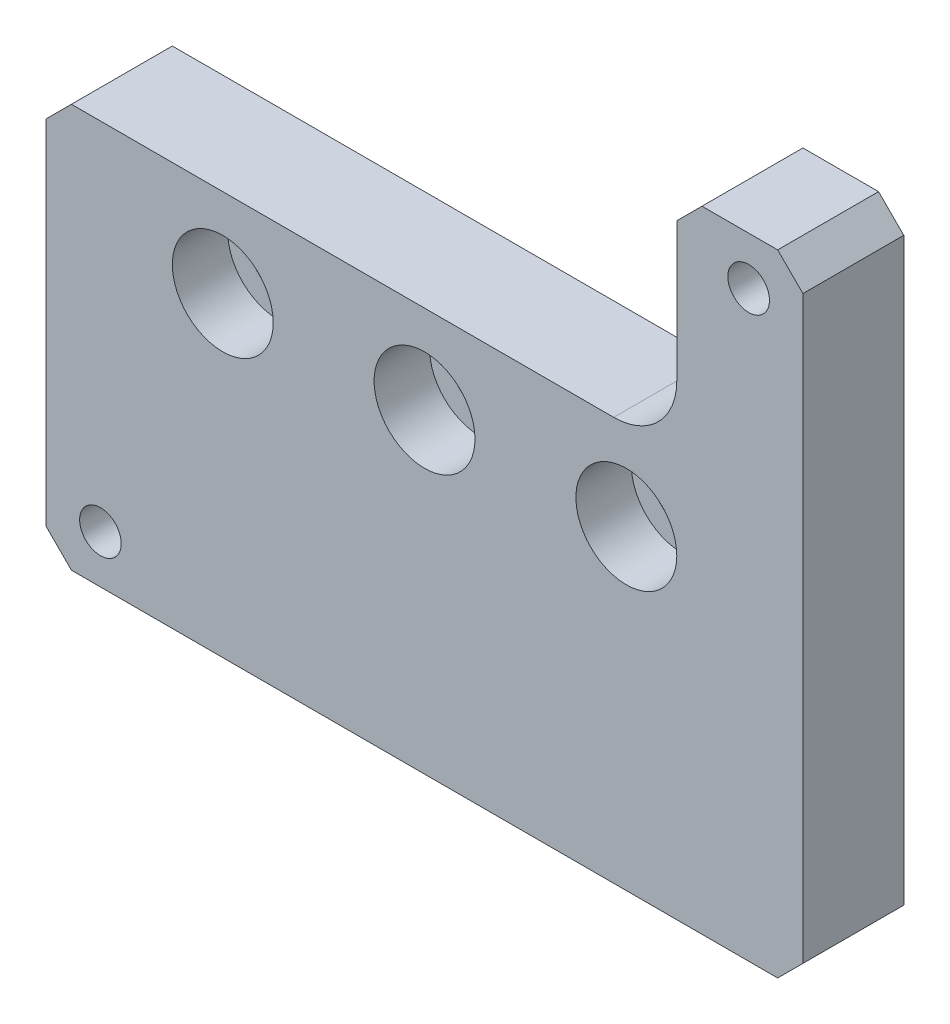
SolidWorks part; units mm, degrees
material "AL6061"
ref_plane "Front Plane" through (0, 0, 0) normal (0, 0, 1) x (1, 0, 0)
ref_plane "Top Plane" through (0, 0, 0) normal (0, 1, 0) x (1, 0, 0)
ref_plane "Right Plane" through (0, 0, 0) normal (1, 0, 0) x (0, 0, -1)
sketch "Sketch1" plane through (0, 0, 0) normal (0, 0, 1) x (1, 0, 0)
  line L1 (0, 0) -> (60, 0)
  line L2 (0, 0) -> (0, 50)
  line L3 (0, 50) -> (60, 50)
  line L4 (60, 0) -> (60, 50)
  dimension "D1" = 50
  dimension "D2" = 60
extrude "Boss-Extrude1" add sketch "Sketch1" along normal blind 8
hole_wizard "CBORE for M4 Hex Socket Head Cap Screw1" positions "Sketch2" profile "Sketch3" counterbore size "M4" standard "ISO" end condition through all
sketch "Sketch2" plane through (0, 0, 8) normal (0, 0, 1) x (1, 0, 0)
  line L1 (0, 25) -> (60, 25) construction
  line L2 (0, 50) -> (0, 0) construction
  line L3 (60, 0) -> (60, 50) construction
  line L6 (30, 50) -> (30, 0) construction
  line L7 (60, 50) -> (0, 50) construction
  line L8 (0, 0) -> (60, 0) construction
  point P20 (30, 25)
  point P22 (14, 25)
  point P25 (46, 25)
  dimension "D1" = 32
sketch "Sketch3" plane through (46, 25, 8) normal (1, 0, 0) x (0, -1, 0)
  line L0 (0, 0) -> (0, 8)
  line L1 (0, 8) -> (2.25, 8)
  line L3 (2.25, 8) -> (2.25, 4.4)
  line L4 (2.25, 4.4) -> (4, 4.4)
  line L5 (4, 4.4) -> (4, 0)
  line L7 (4, 0) -> (0, 0)
  line L11 (0, -6.35) -> (0, 107.95) construction
  dimension "通孔孔直径" = 4.5
  dimension "通孔孔深度" = 8
  dimension "柱形沉头孔直径" = 8
  dimension "柱形沉头孔深度" = 4.4
hole_wizard "M4 Tapped Hole1" positions "Sketch4" profile "Sketch5" tap size "M4" standard "ISO" end condition through all
sketch "Sketch4" plane through (0, 0, 8) normal (0, 0, 1) x (1, 0, 0)
  line L0 (0, 25) -> (60, 25) construction
  line L1 (0, 50) -> (0, 0) construction
  line L2 (60, 0) -> (60, 50) construction
  line L5 (30, 50) -> (30, 0) construction
  line L6 (60, 50) -> (0, 50) construction
  line L7 (0, 0) -> (60, 0) construction
  point P23 (4.3, 3.8)
  point P25 (55.7, 46.2)
  dimension "D1" = 42.4
  dimension "D2" = 21.2
  dimension "D3" = 25.7
  dimension "D4" = 51.4
sketch "Sketch5" plane through (55.7, 46.2, 8) normal (1, 0, 0) x (0, -1, 0)
  line L0 (0, 0) -> (0, 8)
  line L1 (0, 8) -> (1.65, 8)
  line L2 (1.65, 8) -> (1.65, 0)
  line L5 (1.65, 0) -> (0, 0)
  line L11 (0, -6.35) -> (0, 107.95) construction
  dimension "通孔螺纹孔钻头直径" = 3.3
  dimension "通孔螺纹孔钻头深度" = 8
cosmetic thread "Cosmetic Thread5" parameters "D2"=4
cosmetic thread "Cosmetic Thread6" parameters "D2"=4
chamfer "Chamfer1" distance 2 angle 45 4 edges at (60, 50, 4) (60, 0, 4) (0, 0, 4) (0, 50, 4)
sketch "Sketch6" plane through (0, 0, 0) normal (0, 0, -1) x (-1, 0, 0)
  line L1 (-50, 32) -> (0, 32)
  line L2 (-50, 32) -> (-50, 50)
  line L3 (-50, 50) -> (0, 50)
  line L4 (0, 32) -> (0, 50)
  line L7 (-58, 50) -> (-2, 50) construction
  line L8 (0, 48) -> (0, 2) construction
  line L9 (-60, 2) -> (-60, 48) construction
  dimension "D1" = 18
  dimension "D2" = 10
extrude "Cut-Extrude1" cut sketch "Sketch6" against normal through all
chamfer "Chamfer2" distance 2 angle 45 2 edges at (0, 32, 4) (50, 50, 4)
fillet "Fillet1" radius 5 1 edges at (50, 32, 4)
